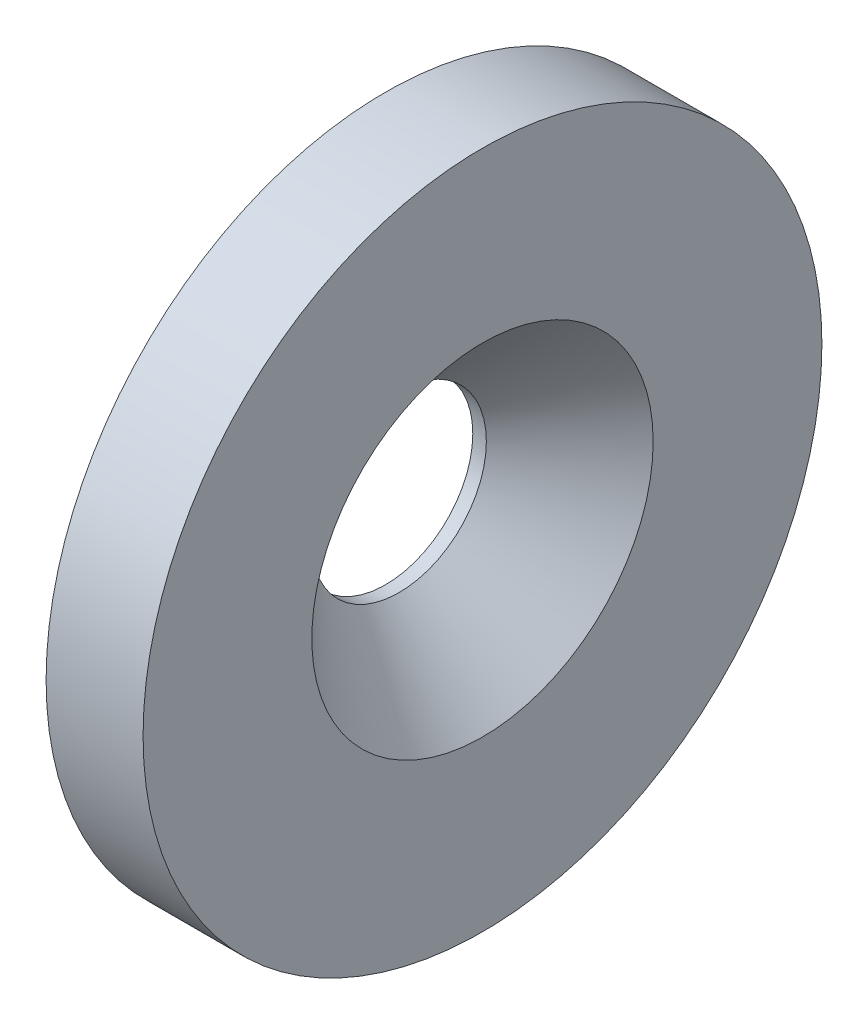
SolidWorks part; units mm, degrees
ref_plane "前视基准面" through (0, 0, 0) normal (0, 0, 1) x (1, 0, 0)
ref_plane "上视基准面" through (0, 0, 0) normal (0, 1, 0) x (1, 0, 0)
ref_plane "右视基准面" through (0, 0, 0) normal (1, 0, 0) x (0, 0, -1)
sketch "草图1" plane through (0, 0, 0) normal (1, 0, 0) x (0, 0, -1)
  circle A0 centre (0, 0) radius 17.5
  dimension "D1" = 35
extrude "凸台-拉伸1" add sketch "草图1" along normal blind 5
hole_wizard "打孔尺寸(%根据)内六角花形沉头螺钉的类型1" positions "草图2" profile "草图3" countersink size "M8" standard "GB" end condition through all
sketch "草图2" plane through (5, 0, 0) normal (1, 0, 0) x (0, 0, -1)
  point P0 (0, 0)
sketch "草图3" plane through (5, 0, 0) normal (0, 1, 0) x (0, 0, -1)
  line L0 (0, 0) -> (0, 5)
  line L1 (0, 5) -> (4.5, 5)
  line L2 (4.5, 5) -> (4.5, 4.3)
  line L3 (4.5, 4.3) -> (8.8, 0)
  line L5 (8.8, 0) -> (0, 0)
  line L6 (-4.5, 4.3) -> (-8.8, 0) construction
  line L11 (0, -6.35) -> (0, 107.95) construction
  dimension "通孔孔直径" = 9
  dimension "通孔孔深度" = 5
  dimension "近端锥形沉头孔直径" = 17.6
  dimension "近端锥形沉头孔角度" = 90
